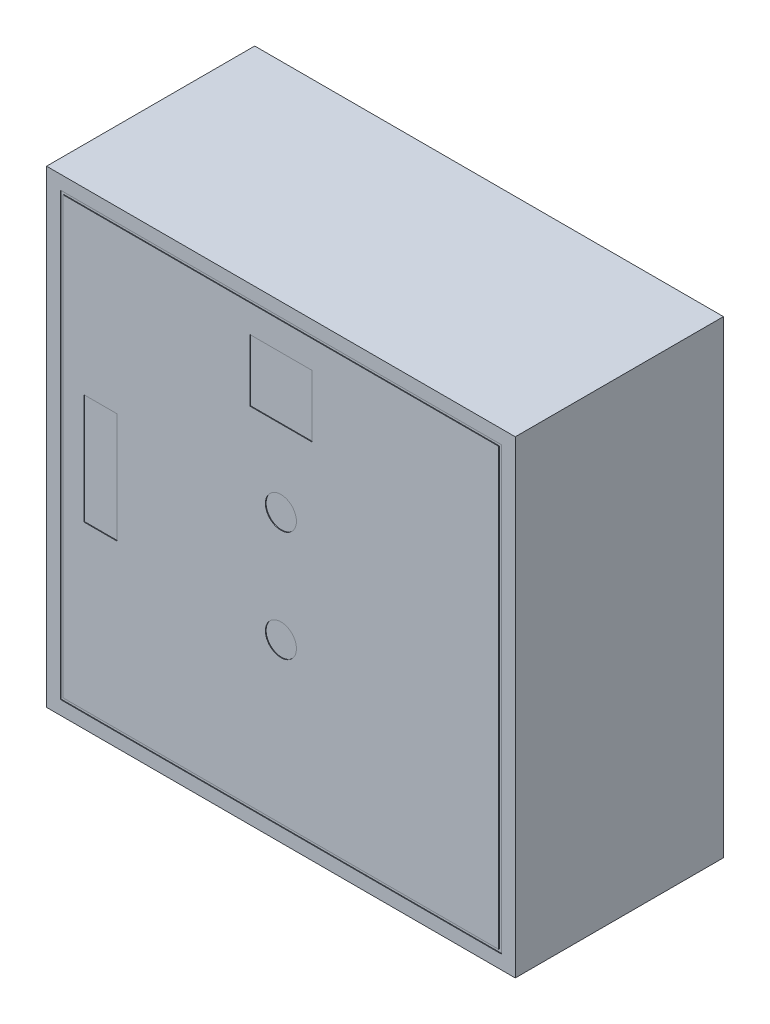
from build123d import *

# Parameters (mm, degrees)
SKETCH1_W           = 340
SKETCH1_H           = 340
BOSS_EXTRUDE1_DEPTH = 150
SHELL1_T            = -1.5
SKETCH2_W           = 340
SKETCH2_H           = 340
BOSS_EXTRUDE2_DEPTH = 1
SKETCH3_W           = 320
SKETCH3_H           = 320
SKETCH3_W_2         = 316
SKETCH3_H_2         = 316
SKETCH3_R           = 11.25
SKETCH3_W_3         = 24
SKETCH3_H_3         = 80
SKETCH3_W_4         = 45
SKETCH3_H_4         = 45
CUT_EXTRUDE1_DEPTH  = 0.5


with BuildPart() as part:
    # Sketch1 → Boss-Extrude1 (new body)
    with BuildSketch(Plane.XY):
        with Locations((170, 170)):
            Rectangle(SKETCH1_W, SKETCH1_H)
    extrude(amount=BOSS_EXTRUDE1_DEPTH)

    # Shell1
    shell1_openings = [part.faces().sort_by_distance(p)[0] for p in [
        (170, 170, 150),
    ]]
    offset(amount=SHELL1_T, openings=shell1_openings, kind=Kind.INTERSECTION)

    # Sketch2 → Boss-Extrude2 (add)
    with BuildSketch(Plane.XY.offset(150)):
        with Locations((170, 170)):
            Rectangle(SKETCH2_W, SKETCH2_H)
    extrude(amount=BOSS_EXTRUDE2_DEPTH)

    # Sketch3 → Cut-Extrude1 (cut)
    # profile 1 of 5: a face of its own
    with BuildSketch(Plane.XY.offset(151)):
        with Locations((170, 170)):
            Rectangle(SKETCH3_W, SKETCH3_H)
        with Locations((170, 170)):
            Rectangle(SKETCH3_W_2, SKETCH3_H_2, mode=Mode.SUBTRACT)
    # profile 2 of 5: a face of its own
    with BuildSketch(Plane.XY.offset(151)):
        with Locations((170, 207.5)):
            Circle(SKETCH3_R)
    # profile 3 of 5: a face of its own
    with BuildSketch(Plane.XY.offset(151)):
        with Locations((170, 127.5)):
            Circle(SKETCH3_R)
    # profile 4 of 5: a face of its own
    with BuildSketch(Plane.XY.offset(151)):
        with Locations((39, 170)):
            Rectangle(SKETCH3_W_3, SKETCH3_H_3)
    # profile 5 of 5: a face of its own
    with BuildSketch(Plane.XY.offset(151)):
        with Locations((170, 285.5)):
            Rectangle(SKETCH3_W_4, SKETCH3_H_4)
    extrude(amount=-CUT_EXTRUDE1_DEPTH, mode=Mode.SUBTRACT)


solid = part.part
